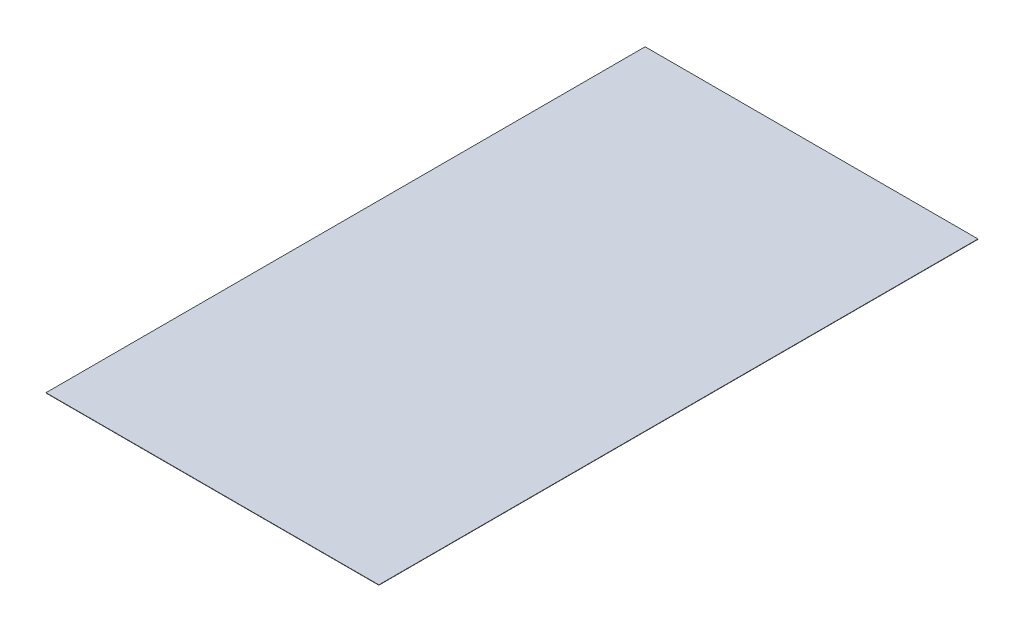
SolidWorks part; units mm, degrees
ref_plane "Front Plane" through (0, 0, 0) normal (0, 0, 1) x (1, 0, 0)
ref_plane "Top Plane" through (0, 0, 0) normal (0, 1, 0) x (1, 0, 0)
ref_plane "Right Plane" through (0, 0, 0) normal (1, 0, 0) x (0, 0, -1)
sketch "Sketch1" plane through (0, 0, 0) normal (0, 1, 0) x (1, 0, 0)
  line L1 (-500, -900) -> (500, -900)
  line L2 (-500, -900) -> (-500, 900)
  line L3 (-500, 900) -> (500, 900)
  line L4 (500, -900) -> (500, 900)
  line L5 (-500, -900) -> (500, 900) construction
  line L6 (-500, 900) -> (500, -900) construction
  point P0 (0, 0)
  dimension "D1" = 1000
  dimension "D2" = 1800
extrude "Boss-Extrude1" add sketch "Sketch1" along normal blind 1
